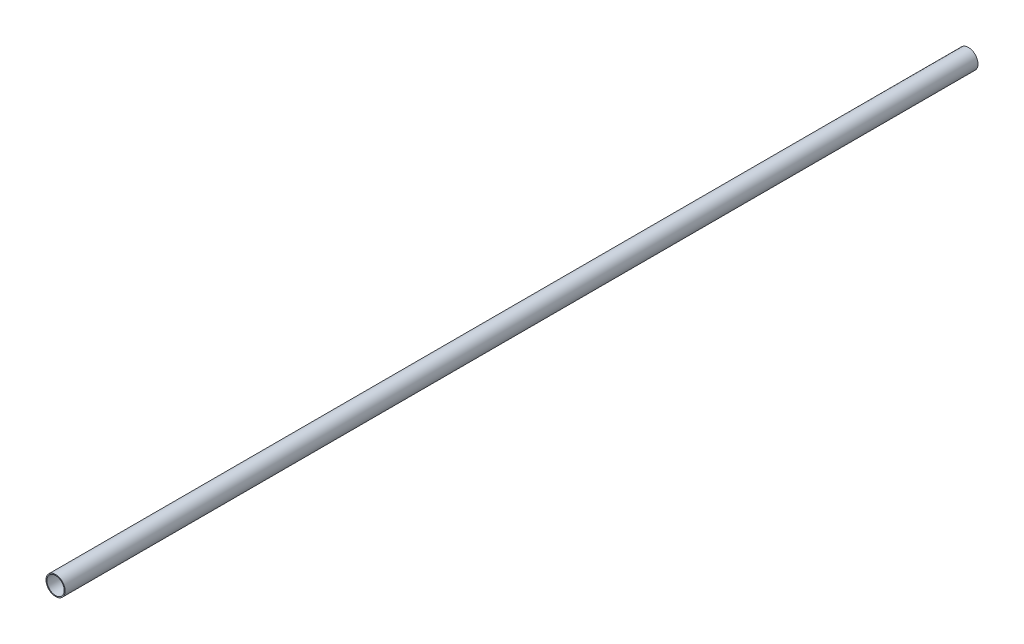
SolidWorks part; units mm, degrees
material "普通碳钢"
ref_plane "Front Plane" through (0, 0, 0) normal (0, 0, 1) x (1, 0, 0)
ref_plane "Top Plane" through (0, 0, 0) normal (0, 1, 0) x (1, 0, 0)
ref_plane "Right Plane" through (0, 0, 0) normal (1, 0, 0) x (0, 0, -1)
sketch "Sketch1" plane through (0, 0, 0) normal (0, 0, 1) x (1, 0, 0)
  circle A0 centre (0, 0) radius 21
  circle A1 centre (0, 0) radius 19
  dimension "D1" = 38
  dimension "D2" = 42
extrude "Boss-Extrude1" add sketch "Sketch1" along normal blind 2000
